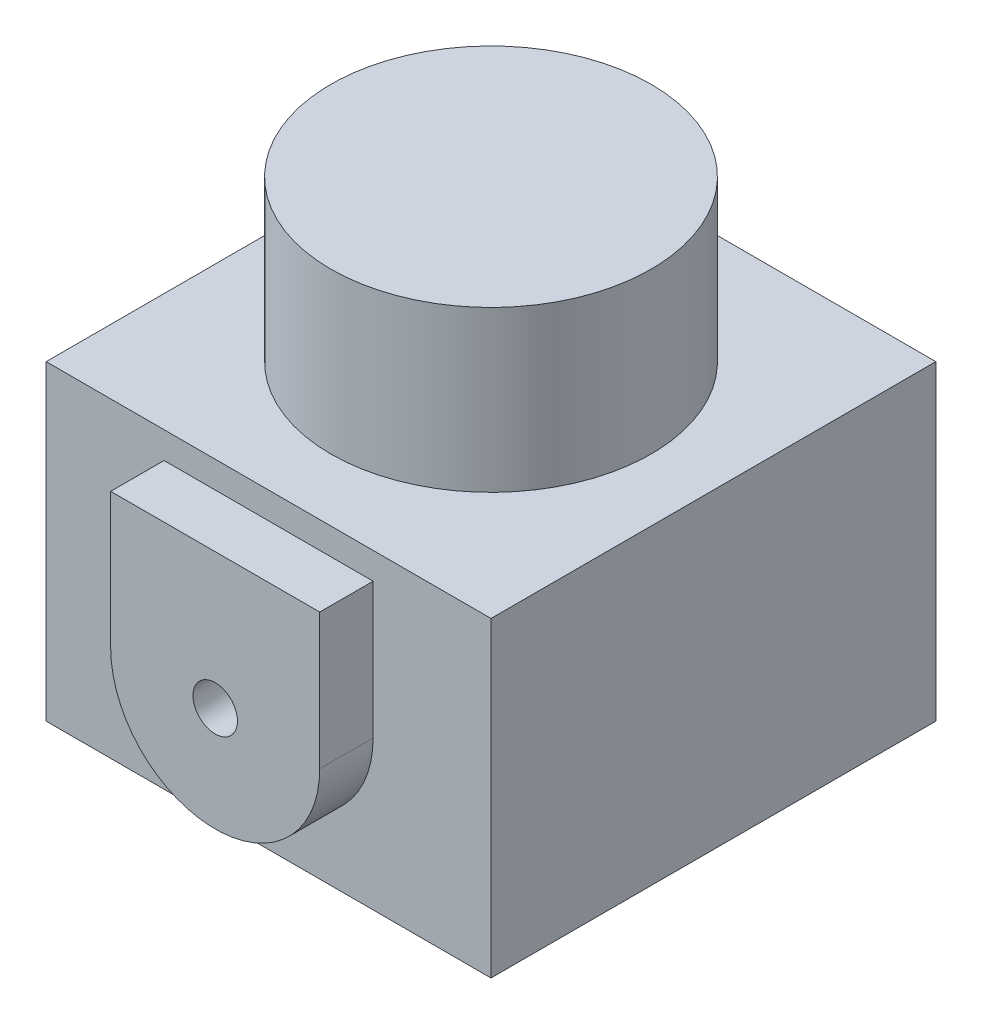
from build123d import *

# Parameters (mm, degrees)
SKETCH1_W             = 50
SKETCH1_H             = 50
BOSS_EXTRUDE1_DEPTH   = 35
SKETCH2_R             = 18
BOSS_EXTRUDE2_DEPTH   = 18
BOSS_EXTRUDE3_DEPTH   = 6
M6_TAPPED_HOLE1_D     = 5
M6_TAPPED_HOLE1_DEPTH = 17
M6_TAPPED_HOLE1_TIP   = 1.502151548


with BuildPart() as part:
    # Sketch1 → Boss-Extrude1 (new body)
    with BuildSketch(Plane(origin=(0, 0, 0), x_dir=(1, 0, 0), z_dir=(0, 1, 0))):
        Rectangle(SKETCH1_W, SKETCH1_H)
    extrude(amount=BOSS_EXTRUDE1_DEPTH)

    # Sketch2 → Boss-Extrude2 (add)
    with BuildSketch(Plane(origin=(0, 35, 0), x_dir=(1, 0, 0), z_dir=(0, 1, 0))):
        with Locations(Location((0, 0, 0), (0, 0, 270))):
            Circle(SKETCH2_R)
    extrude(amount=BOSS_EXTRUDE2_DEPTH)

    # Sketch3 → Boss-Extrude3 (add)
    with BuildSketch(Plane.XY.offset(25)):
        with BuildLine():
            Line((11.75, 32), (-11.75, 32))
            Line((-11.75, 32), (-11.75, 16.75))
            ThreePointArc((-11.75, 16.75), (0, 5), (11.75, 16.75))
            Line((11.75, 16.75), (11.75, 32))
        make_face()
    extrude(amount=BOSS_EXTRUDE3_DEPTH)

    # M6 Tapped Hole1
    with Locations(Plane.XY.offset(31)):
        with Locations((0, 16.75)):
            Hole(M6_TAPPED_HOLE1_D / 2, depth=M6_TAPPED_HOLE1_DEPTH)
            with Locations((0, 0, -(M6_TAPPED_HOLE1_DEPTH + M6_TAPPED_HOLE1_TIP / 2))):  # 118° drill point
                Cone(0, M6_TAPPED_HOLE1_D / 2, M6_TAPPED_HOLE1_TIP, mode=Mode.SUBTRACT)


solid = part.part
